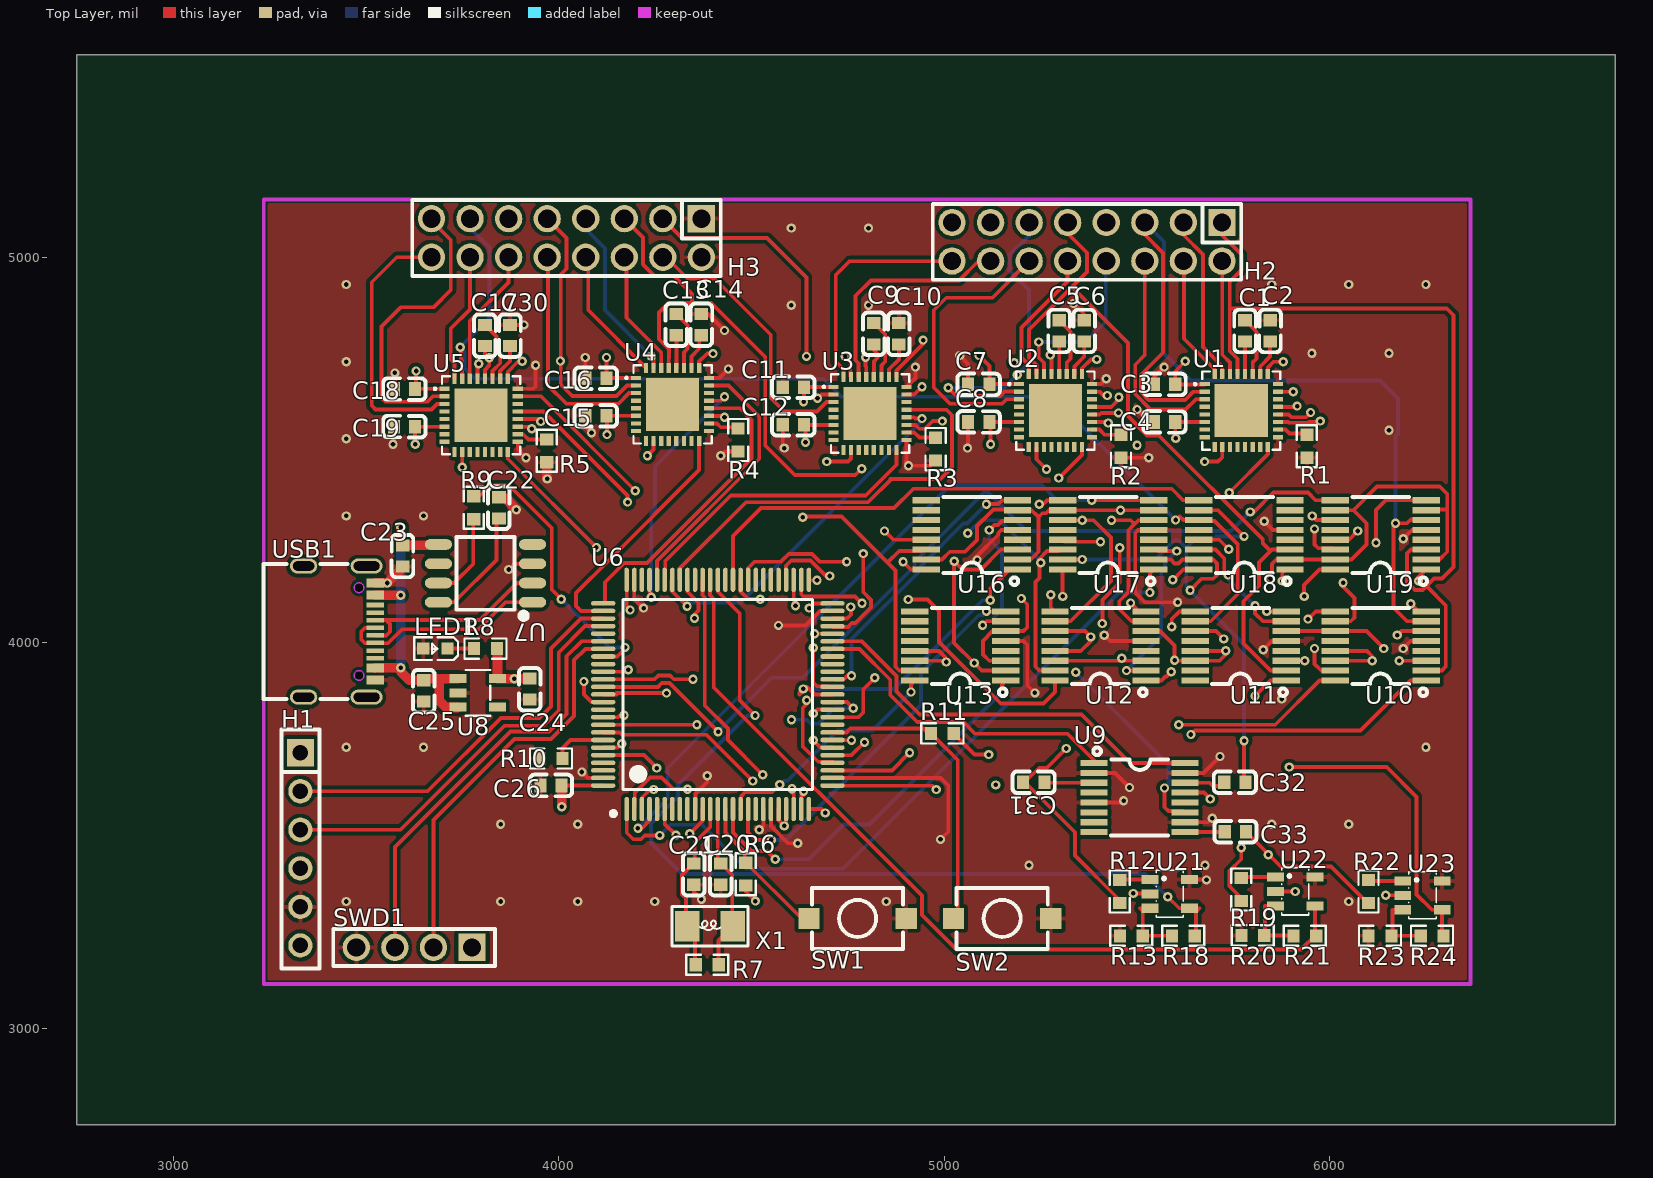
[diagram p0: Top Layer view]
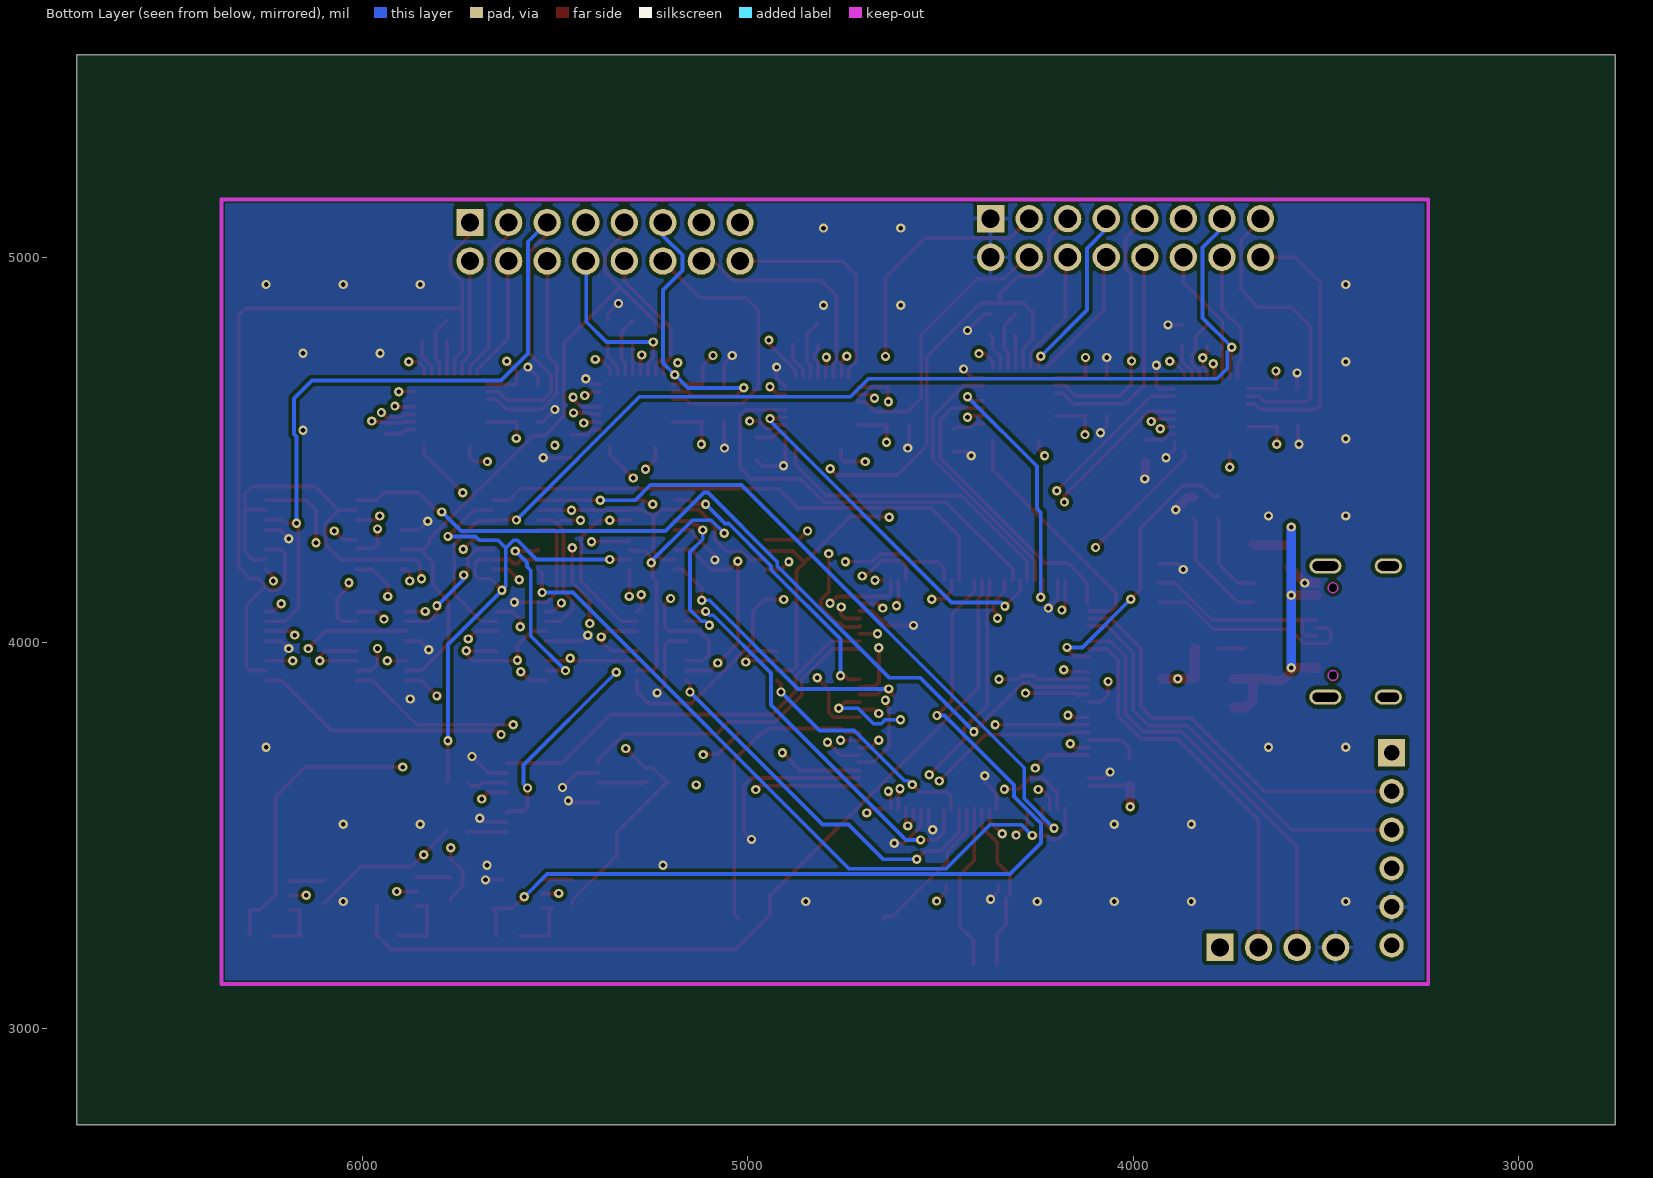
[diagram p1: Bottom Layer view, seen from below]
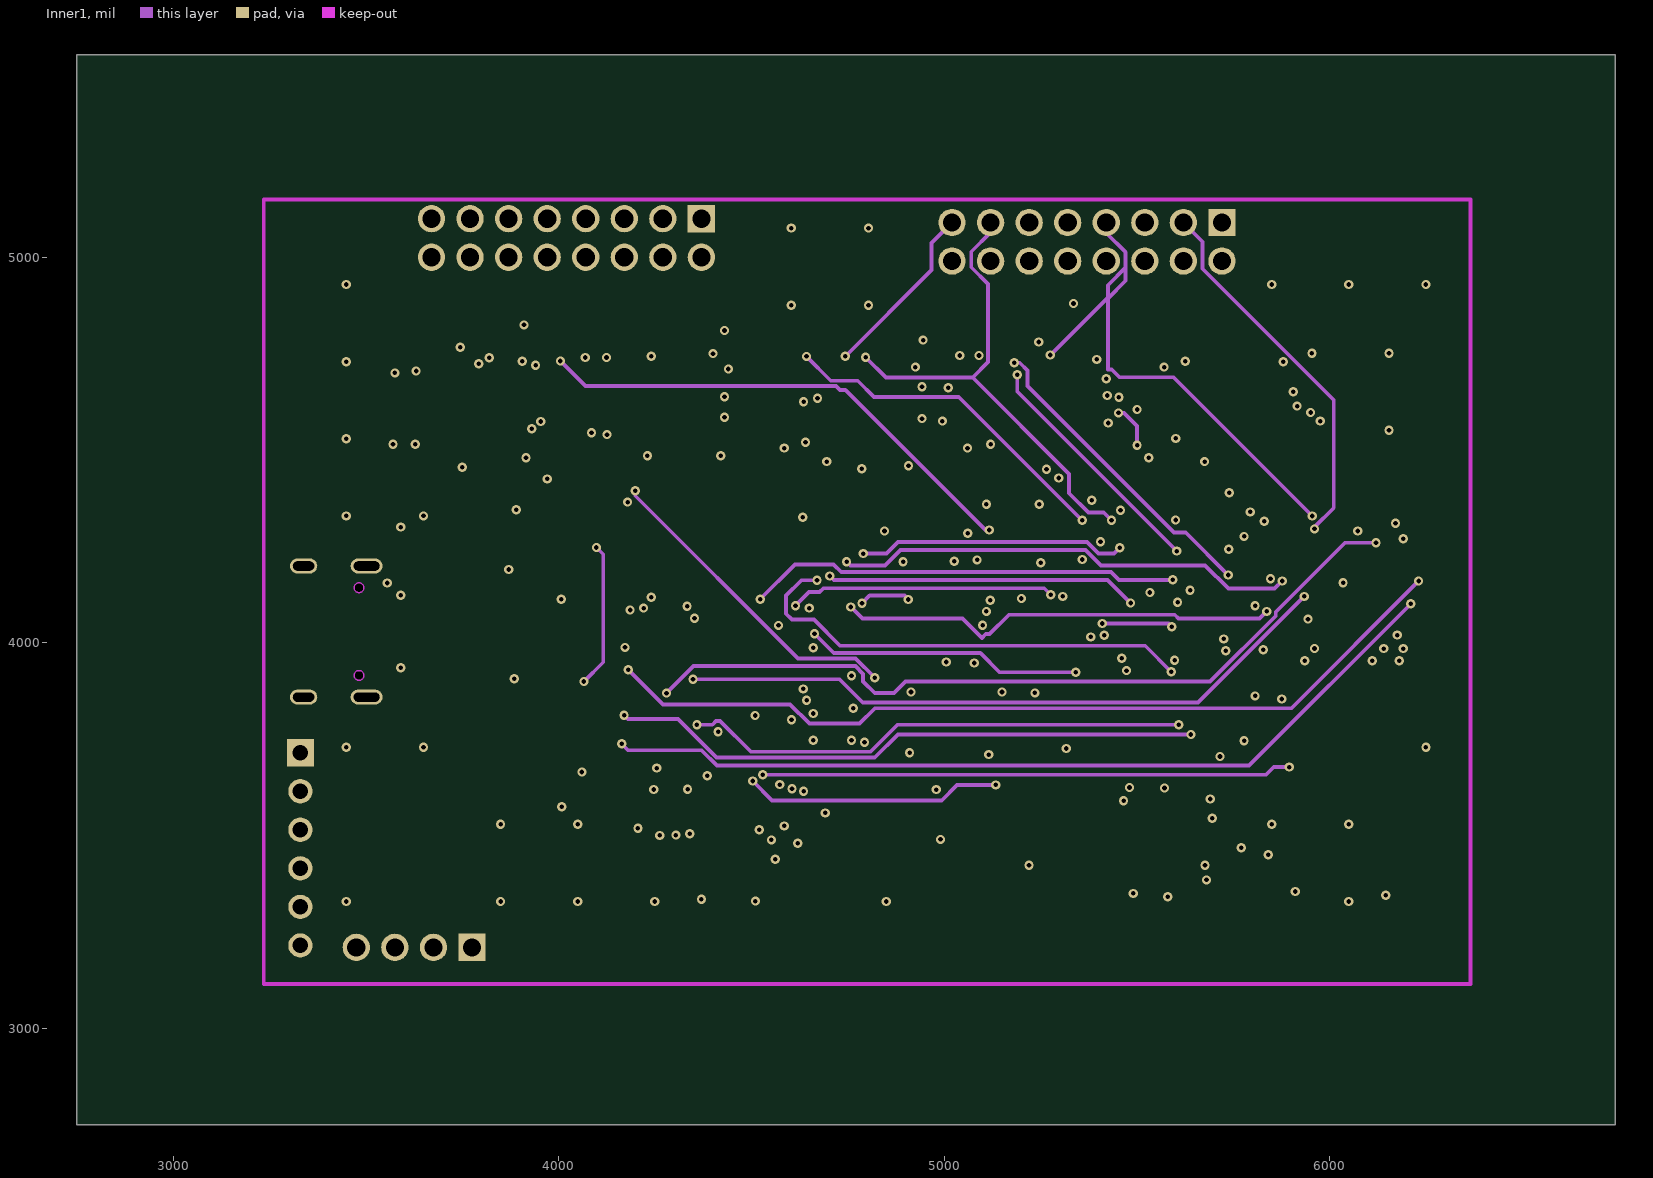
[diagram p2: Inner1]
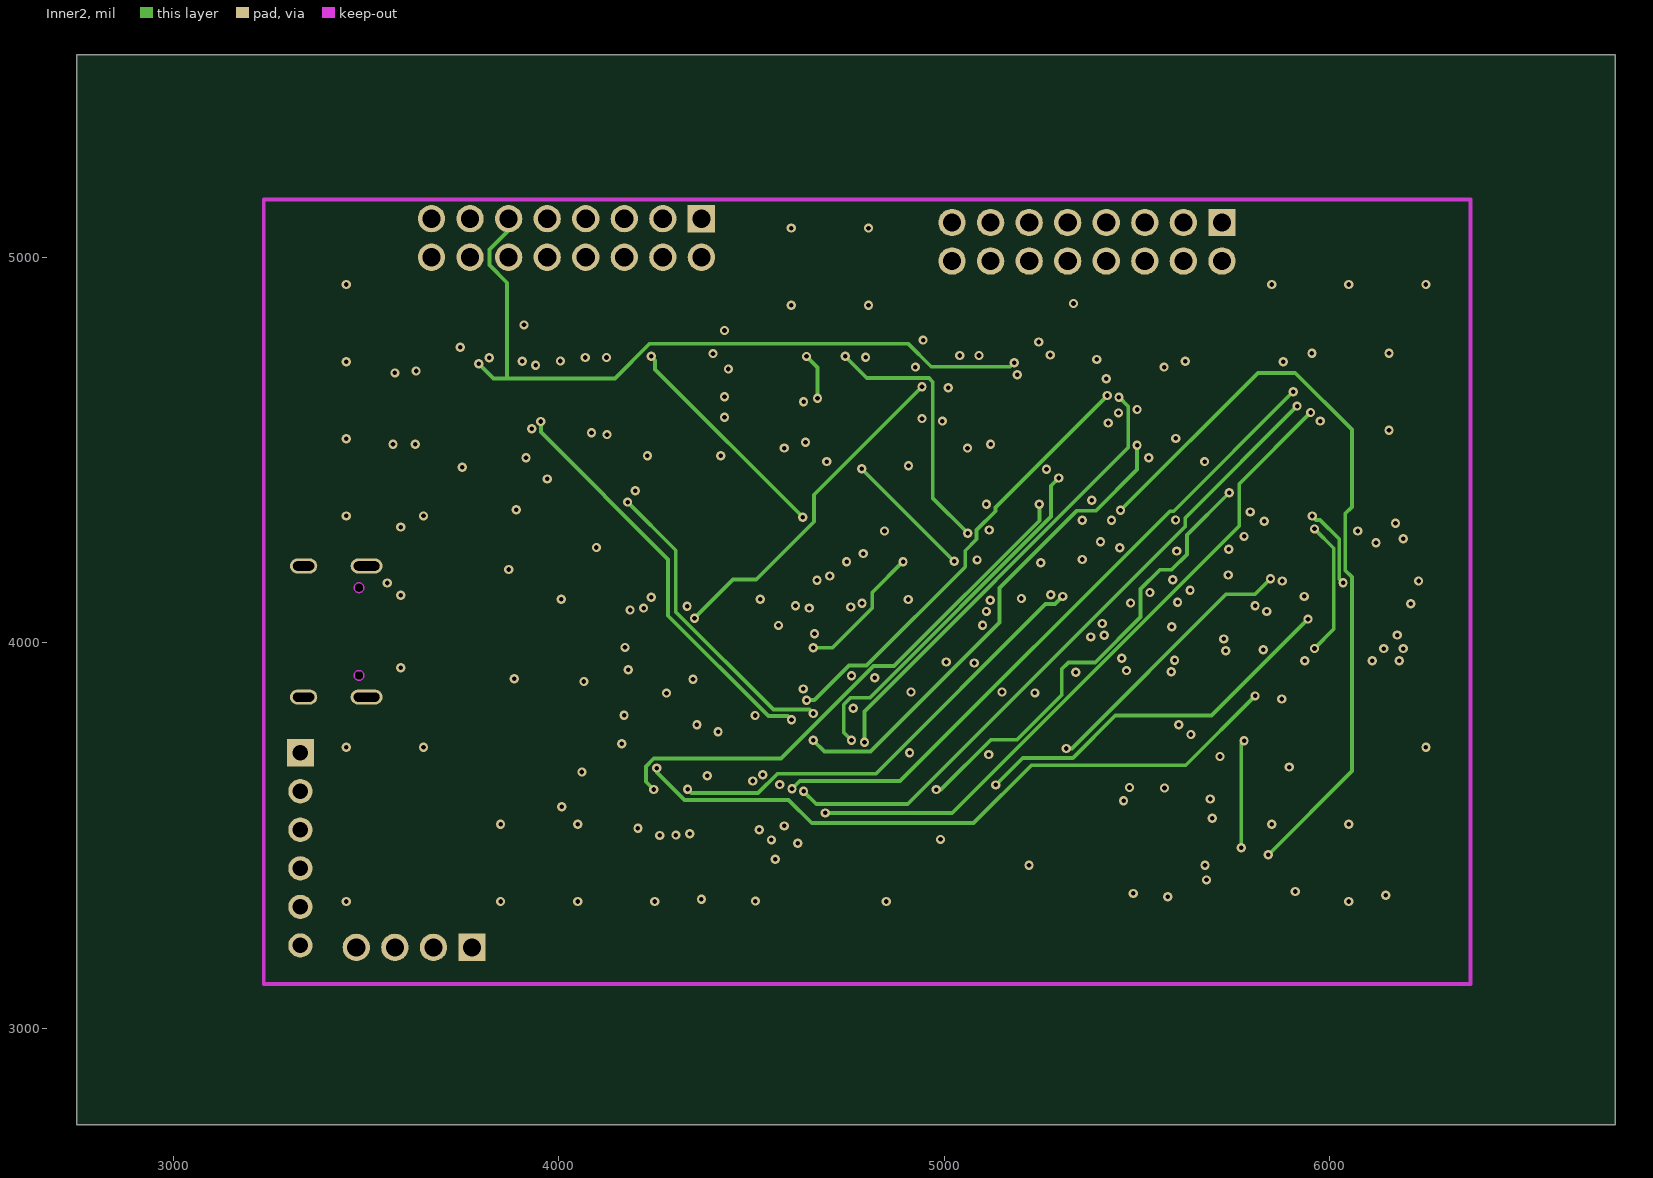
[diagram p3: Inner2]
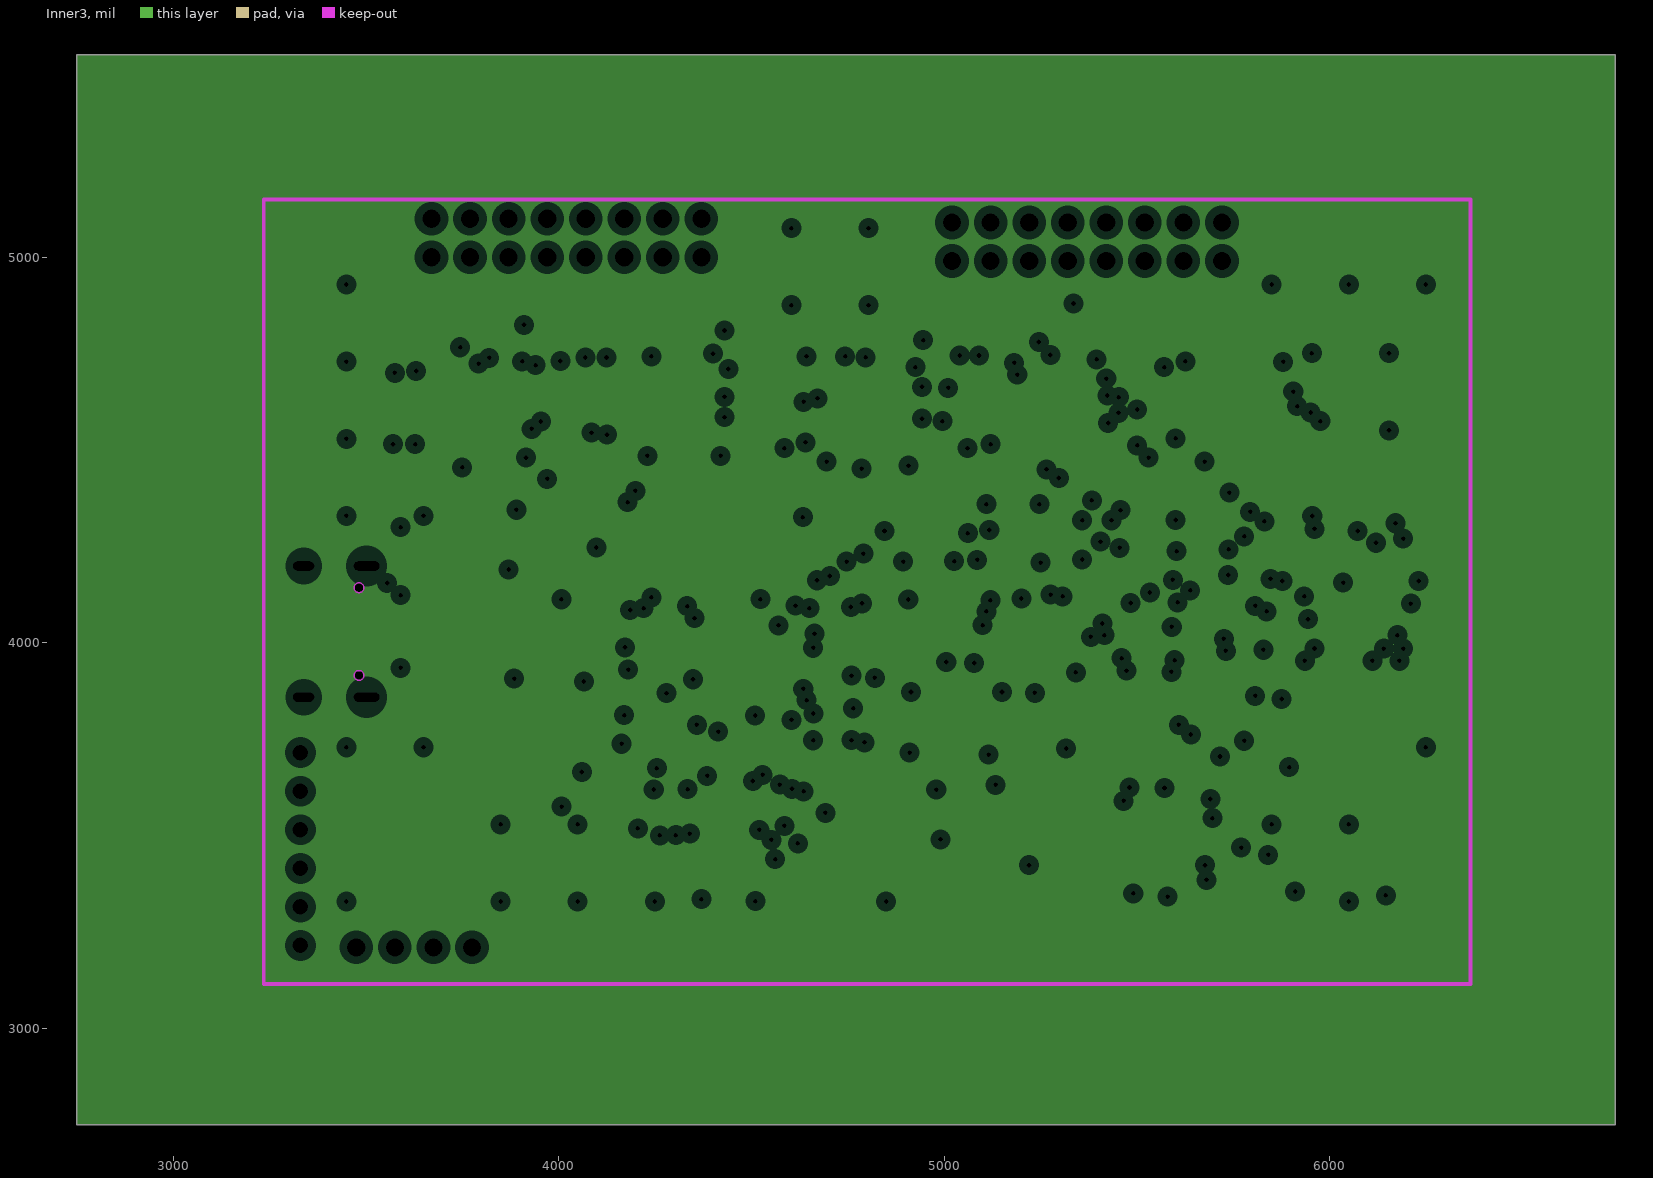
[diagram p4: Inner3, clearances drawn from the general rule]
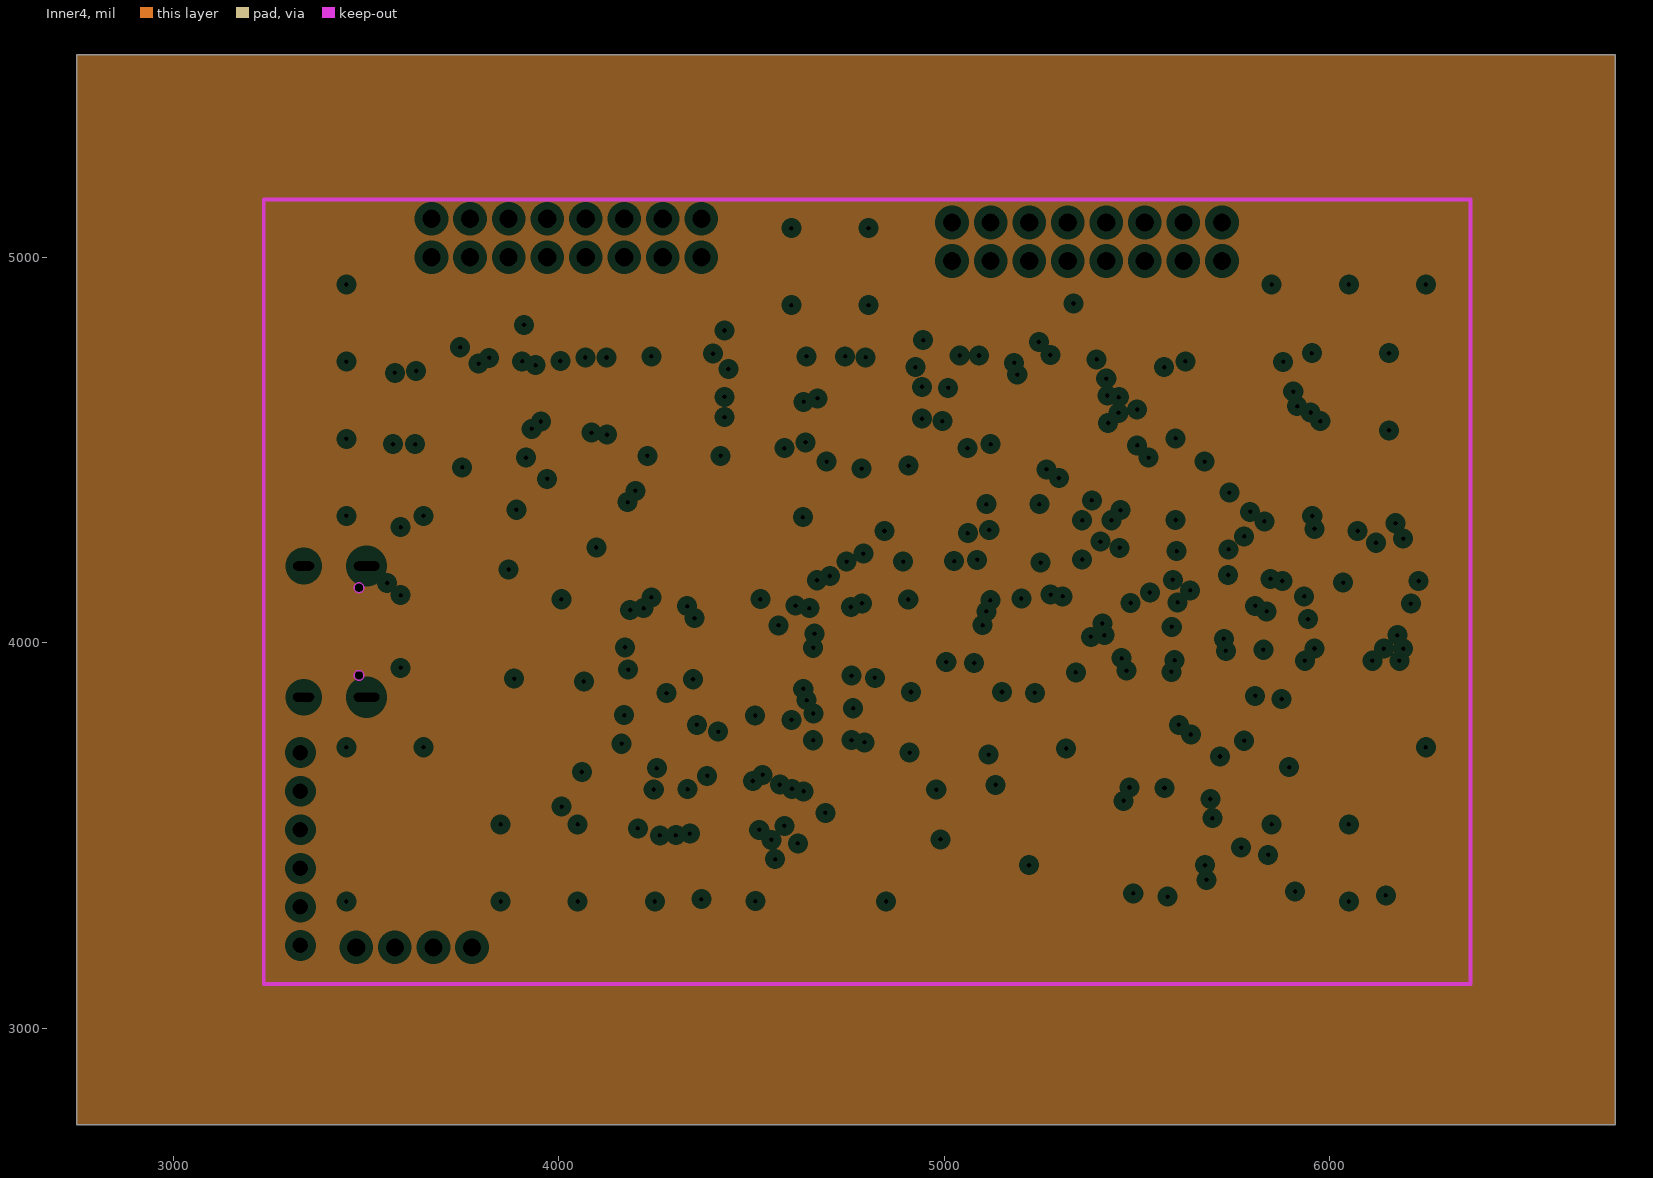
[diagram p5: Inner4, clearances drawn from the general rule]
# Altium PCB MISC49858.pcbdoc (part 1 of 3)
Units mil, origin at the board's own origin, x right, y up, seen from the top; angles counter-clockwise.
Board outline 3990 x 2775 mil, 6 copper layers (Top Layer, Inner1, Inner2, Inner3, Inner4, Bottom Layer), stack 60.565 mil thick; 79 components, 151 nets, 603 pads, 275 vias.

## Layer stack, top to bottom
Top Layer: signal copper 1.378
Dielectric1: surface 3.913, 3313 RC57% 4.2mil, Dk 0
Inner1: signal copper 0.598
Dielectric2: surface 21.654, 0.55mm H/H No copper, Dk 0
Inner2: signal copper 0.598
Dielectric3: surface 4.283, 2116 RC54% 4.9mil, Dk 0
Inner3: plane copper 0.598
Dielectric4: surface 21.654, 0.55mm H/H No copper, Dk 0
Inner4: plane copper 0.598
Dielectric5: surface 3.913, 3313 RC57% 4.2mil, Dk 0
Bottom Layer: signal copper 1.378

## Board outline
6740,2750 2750,2750 2750,5525 6740,5525

## Design rules (kind name [scope] priority, off if disabled: settings)
BoardOutlineClearance copperThickness2oz_1 [All] p2 off: genericclearance=7.99 ignorepadtopadclearanceinfootprint=FALSE except(0: Arc-SplitContinuation Track-SplitContinuation SMDPad-SplitContinuation THPad-SplitContinuation Via-SplitContinuation Fill-SplitContinuation Region-SplitContinuation Poly-SplitContinuation Text-SplitContinuation Hole-SplitContinuation; 5.98: SMDPad-CutoutEdge THPad-CutoutEdge Via-CutoutEdge Fill-CutoutEdge Region-CutoutEdge Text-CutoutEdge Hole-CutoutEdge; 10: Poly-OutlineEdge Poly-CutoutEdge; 11.81: Arc-OutlineEdge Track-OutlineEdge SMDPad-OutlineEdge THPad-OutlineEdge Via-OutlineEdge Fill-OutlineEdge Region-OutlineEdge Text-OutlineEdge Hole-OutlineEdge Arc-CutoutEdge Track-CutoutEdge)
BoardOutlineClearance Plane_innerPlane_1 [All] p4 off: genericclearance=4.02 ignorepadtopadclearanceinfootprint=FALSE except(0: Arc-SplitContinuation Track-SplitContinuation SMDPad-SplitContinuation THPad-SplitContinuation Via-SplitContinuation Fill-SplitContinuation Region-SplitContinuation Poly-SplitContinuation Text-SplitContinuation Hole-SplitContinuation; 5.98: SMDPad-CutoutEdge THPad-CutoutEdge Via-CutoutEdge Fill-CutoutEdge Region-CutoutEdge Text-CutoutEdge Hole-CutoutEdge; 10: Poly-OutlineEdge Poly-CutoutEdge; 11.81: Arc-OutlineEdge Track-OutlineEdge SMDPad-OutlineEdge THPad-OutlineEdge Via-OutlineEdge Fill-OutlineEdge Region-OutlineEdge Text-OutlineEdge Hole-OutlineEdge Arc-CutoutEdge Track-CutoutEdge)
BoardOutlineClearance Copper_copperRegion_1 [All] p6 off: genericclearance=4.02 ignorepadtopadclearanceinfootprint=FALSE except(0: Arc-SplitContinuation Track-SplitContinuation SMDPad-SplitContinuation THPad-SplitContinuation Via-SplitContinuation Fill-SplitContinuation Region-SplitContinuation Poly-SplitContinuation Text-SplitContinuation Hole-SplitContinuation; 5.98: SMDPad-CutoutEdge THPad-CutoutEdge Via-CutoutEdge Fill-CutoutEdge Region-CutoutEdge Text-CutoutEdge Hole-CutoutEdge; 10: Poly-OutlineEdge Poly-CutoutEdge; 11.81: Arc-OutlineEdge Track-OutlineEdge SMDPad-OutlineEdge THPad-OutlineEdge Via-OutlineEdge Fill-OutlineEdge Region-OutlineEdge Text-OutlineEdge Hole-OutlineEdge Arc-CutoutEdge Track-CutoutEdge)
BoardOutlineClearance copperThickness1oz_1 [All] p8: genericclearance=4.02 ignorepadtopadclearanceinfootprint=FALSE except(0: Arc-SplitContinuation Track-SplitContinuation SMDPad-SplitContinuation THPad-SplitContinuation Via-SplitContinuation Fill-SplitContinuation Region-SplitContinuation Poly-SplitContinuation Text-SplitContinuation Hole-SplitContinuation; 5.98: SMDPad-CutoutEdge THPad-CutoutEdge Via-CutoutEdge Fill-CutoutEdge Region-CutoutEdge Text-CutoutEdge Hole-CutoutEdge; 10: Poly-OutlineEdge Poly-CutoutEdge; 11.81: Arc-OutlineEdge Track-OutlineEdge SMDPad-OutlineEdge THPad-OutlineEdge Via-OutlineEdge Fill-OutlineEdge Region-OutlineEdge Text-OutlineEdge Hole-OutlineEdge Arc-CutoutEdge Track-CutoutEdge)
Clearance copperThickness2oz [All] p1 off: gap=7.99 ignorepadtopadclearanceinfootprint=FALSE except(5.98: SMDPad-Track SMDPad-SMDPad THPad-Track SMDPad-THPad THPad-THPad Track-Via SMDPad-Via THPad-Via Via-Via Fill-Track Region-Track Fill-SMDPad Region-SMDPad Fill-THPad Region-THPad Fill-Via Region-Via Fill-Fill Fill-Region Region-Region Arc-Track Arc-SMDPad Arc-THPad Arc-Via Fill-Arc Region-Arc Arc-Arc Text-Track SMDPad-Text Text-THPad Text-Via Fill-Text Region-Text Arc-Text Text-Text Hole-Track Hole-SMDPad Hole-THPad Hole-Via Fill-Hole Region-Hole Hole-Arc Hole-Text; 10: Poly-Track Poly-SMDPad Poly-THPad Poly-Via Poly-Fill Poly-Region Poly-Poly Poly-Arc Poly-Text Poly-Hole)
Clearance Plane_innerPlane [All] p3 off: gap=4.02 ignorepadtopadclearanceinfootprint=FALSE except(5.98: SMDPad-Track SMDPad-SMDPad THPad-Track SMDPad-THPad THPad-THPad Track-Via SMDPad-Via THPad-Via Via-Via Fill-Track Region-Track Fill-SMDPad Region-SMDPad Fill-THPad Region-THPad Fill-Via Region-Via Fill-Fill Fill-Region Region-Region Arc-Track Arc-SMDPad Arc-THPad Arc-Via Fill-Arc Region-Arc Arc-Arc Text-Track SMDPad-Text Text-THPad Text-Via Fill-Text Region-Text Arc-Text Text-Text Hole-Track Hole-SMDPad Hole-THPad Hole-Via Fill-Hole Region-Hole Hole-Arc Hole-Text; 10: Poly-Track Poly-SMDPad Poly-THPad Poly-Via Poly-Fill Poly-Region Poly-Poly Poly-Arc Poly-Text Poly-Hole)
Clearance Copper_copperRegion [All] p5 off: gap=4.02 ignorepadtopadclearanceinfootprint=FALSE except(5.98: SMDPad-Track SMDPad-SMDPad THPad-Track SMDPad-THPad THPad-THPad Track-Via SMDPad-Via THPad-Via Via-Via Fill-Track Region-Track Fill-SMDPad Region-SMDPad Fill-THPad Region-THPad Fill-Via Region-Via Fill-Fill Fill-Region Region-Region Arc-Track Arc-SMDPad Arc-THPad Arc-Via Fill-Arc Region-Arc Arc-Arc Text-Track SMDPad-Text Text-THPad Text-Via Fill-Text Region-Text Arc-Text Text-Text Hole-Track Hole-SMDPad Hole-THPad Hole-Via Fill-Hole Region-Hole Hole-Arc Hole-Text; 10: Poly-Track Poly-SMDPad Poly-THPad Poly-Via Poly-Fill Poly-Region Poly-Poly Poly-Arc Poly-Text Poly-Hole)
Clearance copperThickness1oz [All] p7: gap=4.02 ignorepadtopadclearanceinfootprint=FALSE except(5.98: SMDPad-Track SMDPad-SMDPad THPad-Track SMDPad-THPad THPad-THPad Track-Via SMDPad-Via THPad-Via Via-Via Fill-Track Region-Track Fill-SMDPad Region-SMDPad Fill-THPad Region-THPad Fill-Via Region-Via Fill-Fill Fill-Region Region-Region Arc-Track Arc-SMDPad Arc-THPad Arc-Via Fill-Arc Region-Arc Arc-Arc Text-Track SMDPad-Text Text-THPad Text-Via Fill-Text Region-Text Arc-Text Text-Text Hole-Track Hole-SMDPad Hole-THPad Hole-Via Fill-Hole Region-Hole Hole-Arc Hole-Text; 10: Poly-Track Poly-SMDPad Poly-THPad Poly-Via Poly-Fill Poly-Region Poly-Poly Poly-Arc Poly-Text Poly-Hole)
DiffPairsRouting differentialPair [All] p1: maxlimit=6 minlimit=6 mostfreqgap=6 toplayer_minwidth=5 toplayer_prefwidth=10 toplayer_maxwidth=100 toplayer_mingap=6 toplayer_prefgap=6 toplayer_maxgap=6 midlayer1_minwidth=5 midlayer1_prefwidth=10 midlayer1_maxwidth=100 midlayer1_mingap=6 midlayer1_prefgap=6 midlayer1_maxgap=6 midlayer2_minwidth=5 midlayer2_prefwidth=10 midlayer2_maxwidth=100 midlayer2_mingap=6 midlayer2_prefgap=6 midlayer2_maxgap=6 bottomlayer_minwidth=5 bottomlayer_prefwidth=10 bottomlayer_maxwidth=100 bottomlayer_mingap=6 bottomlayer_prefgap=6 bottomlayer_maxgap=6 maxuncoupledlength=10
HoleToHoleClearance otherClearance [All] p1: gap=11.8 allowstackedmicrovias=TRUE
Length netLength [All] p1: minlimit=0 maxlimit=0
PasteMaskExpansion pasteMaskExpansion [All] p1: expansion=0
PlaneConnect innerPlane [All] p1: planeconnectstyle=Relief reliefexpansion=20 reliefentries=4 reliefconductorwidth=10 reliefairgap=10
PolygonConnect copperRegion [(InNet('GND'))] p1: connectstyle=Relief reliefconductorwidth=10 reliefentries=4 polygonreliefangle="90 Angle" airgapwidth=10 via.connectstyle=Relief via.reliefconductorwidth=10 via.reliefentries=4 via.polygonreliefangle="90 Angle" via.airgapwidth=10
RoutingVias viaSize [All] p1: holewidth=12.01 width=24.02 viastyle="Through Hole" minholewidth=11.81 minwidth=19.68 maxholewidth=248.03 maxwidth=393.7
SolderMaskExpansion solderMaskExpansion [IsVia] p1: expansion=-1000 istentingtop=TRUE
SolderMaskExpansion solderMaskExpansion [All] p2: expansion=2 istentingtop=FALSE
Width copperThickness2oz_2 [All] p1 off: maxlimit=100 minlimit=8 preferedwidth=10
Width copperThickness1oz_2 [All] p2: maxlimit=100 minlimit=5 preferedwidth=10

## Components (designator, comment, footprint, x,y, rotation, side; value= is the part's Value field where it differs from the comment)
C1 "22pf/50V" C0603#1 5779.97,4809 r90 top
C2 "104" C0603#1 5844.97,4809 r90 top
C3 "10nF/25V" C0603#1 5571.38,4670.11 r0 top
C4 "4.7uF/50V" C0603#1 5571.38,4572.67 r0 top
C5 "4.7uF/50V" C0603#1 5297.87,4809 r90 top
C6 "104" C0603#1 5362.87,4809 r90 top
C7 "4.7uF/50V" C0603#1 5089.27,4670.11 r0 top
C8 "10nF/25V" C0603#1 5089.28,4572.67 r0 top
C9 "4.7uF/50V" C0603#1 4817.14,4801.62 r90 top
C10 "104" C0603#1 4882.14,4801.62 r90 top
C11 "4.7uF/50V" C0603#1 4608.55,4662.73 r0 top
C12 "10nF/25V" C0603#1 4608.55,4565.29 r0 top
C13 "4.7uF/50V" C0603#1 4305,4825 r90 top
C14 "104" C0603#1 4370,4825 r90 top
C15 "4.7uF/50V" C0603#1 4096.41,4588.67 r0 top
C16 "10nF/25V" C0603#1 4096.41,4686.11 r0 top
C17 "4.7uF/50V" C0603#1 3808.59,4796.94 r90 top
C18 "4.7uF/50V" C0603#1 3600,4658.05 r0 top
C19 "10nF/25V" C0603#1 3600,4560.61 r0 top
C20 "22pf" C0603#1 4420,3400 r90 top
C21 "22pf" C0603#1 4350,3400 r90 top
C22 "0.1UF" C0603#2 3845,4350 r90 top
C23 "0.1UF" C0603#2 3595,4225 r90 top
C24 "106" C0603#1 3925,3880 r90 top
C25 "106" C0603#1 3650,3875.12 r90 top
C26 "100nF" C0603#1 3980,3630 r0 top
C30 "104" C0603#1 3873.59,4796.94 r90 top
C31 "500uF" C0603#1 5231.81,3638.55 r180 top
C32 "500uF" C0603#1 5753.49,3638.55 r180 top
C33 "500uF" C0603#1 5755,3510 r180 top
H1 "" HDR-TH_6P-P2.54-V-F 3330,3465 r270 top
H2 "PZ254V-12-16P" HDR-TH_16P-P2.54-V-M-R2-C8-S2.54 5370,5040 r180 top
H3 "PZ254V-12-16P" HDR-TH_16P-P2.54-V-M-R2-C8-S2.54 4020,5050 r180 top
LED1 "19-217/R6C-AL1M2VY/3T" LED0603-RD 3680,3985 r180 top
R1 "470K/1%" R0603 5940.19,4509.77 r90 top
R2 "470K/1%" R0603 5458.08,4509.77 r90 top
R3 "470K/1%" R0603 4977.36,4502.39 r90 top
R4 "470K/1%" R0603 4465.22,4525.77 r90 top
R5 "470K/1%" R0603 3968.81,4497.71 r90 top
R6 "4.7k" R0603 4485,3400 r270 top
R7 "1M" R0603 4385,3165 r180 top
R8 "4.7k" R0603 3810,3985 r0 top
R9 "100R" R0603 3779.66,4350.34 r90 top
R10 "10K" R0603 3980,3700 r180 top
R11 "4.7k" R0603 4995,3765 r0 top
R12 "10K" R0603 5455,3355 r90 top
R13 "10K" R0603 5485,3240 r0 top
R18 "10K" R0603 5620,3240 r0 top
R19 "10K" R0603 5770,3360 r90 top
R20 "10K" R0603 5800.26,3241.02 r0 top
R21 "10K" R0603 5935,3240 r0 top
R22 "10K" R0603 6100,3355 r90 top
R23 "10K" R0603 6130,3240 r0 top
R24 "10K" R0603 6265,3240 r0 top
SW1 "YTS1C0191ABG00" SW-SMD_L6.0-W4.0-LS7.2 4775,3285 r180 top
SW2 "YTS1C0191ABG00" SW-SMD_L6.0-W4.0-LS7.2 5150,3285 r180 top
SWD1 "A2541HWV-4P" HDR-TH_4P-P2.54-V_A2541HWV-4P 3625,3210 r180 top
U1 "PCAP01AD" VQFN-32_L5.0-W5.0-P0.50-TL-EP 5770.19,4602.06 r0 top
U2 "PCAP01AD" VQFN-32_L5.0-W5.0-P0.50-TL-EP 5288.08,4602.06 r0 top
U3 "PCAP01AD" VQFN-32_L5.0-W5.0-P0.50-TL-EP 4807.36,4594.68 r0 top
U4 "PCAP01AD" VQFN-32_L5.0-W5.0-P0.50-TL-EP 4295.22,4618.06 r0 top
U5 "PCAP01AD" VQFN-32_L5.0-W5.0-P0.50-TL-EP 3798.81,4590 r0 top
U6 "STM32F103VET6" LQFP-100_L14.0-W14.0-P0.50-LS16.0-BL 4412.53,3865.99 r0 top
U7 "CH340N" SOP-8_150MIL 3810,4180 r180 top
U8 "RT9013-3.3GB" SOT-23-5_L2.9-W1.6-P0.94-LS2.8-BL 3790,3870 r270 top
U9 "TMUX1112PWR" TSSOP-16_L5.0-W4.4-P0.65-LS6.4-TL 5506.22,3598.55 r0 top
U10 "TMUX1112PWR" TSSOP-16_L5.0-W4.4-P0.65-LS6.4-TL 6131.88,3991.8 r180 top
U11 "TMUX1112PWR" TSSOP-16_L5.0-W4.4-P0.65-LS6.4-TL 5768.46,3991.8 r180 top
U12 "TMUX1112PWR" TSSOP-16_L5.0-W4.4-P0.65-LS6.4-TL 5405.04,3991.8 r180 top
U13 "TMUX1112PWR" TSSOP-16_L5.0-W4.4-P0.65-LS6.4-TL 5041.62,3991.8 r180 top
U16 "TMUX1112PWR" TSSOP-16_L5.0-W4.4-P0.65-LS6.4-TL 5071.62,4279.91 r180 top
U17 "TMUX1112PWR" TSSOP-16_L5.0-W4.4-P0.65-LS6.4-TL 5425.04,4279.91 r180 top
U18 "TMUX1112PWR" TSSOP-16_L5.0-W4.4-P0.65-LS6.4-TL 5778.46,4279.91 r180 top
U19 "TMUX1112PWR" TSSOP-16_L5.0-W4.4-P0.65-LS6.4-TL 6131.88,4279.91 r180 top
U21 "LMV321IDBVR" SOT-23-5_L3.0-W1.7-P0.95-LS2.8-BR 5584.72,3348.85 r180 top
U22 "LMV321IDBVR" SOT-23-5_L3.0-W1.7-P0.95-LS2.8-BR 5910,3355 r180 top
U23 "LMV321IDBVR" SOT-23-5_L3.0-W1.7-P0.95-LS2.8-BR 6240,3345 r180 top
USB1 "TYPE-C16PIN" USB-C-SMD_TYPE-C16PIN 3431.28,4029.1 r270 top
X1 "8MHz" SMD322522 4451.22,3265 r180 top

## Footprints (in the part's own frame and the unit in brackets; to place one, negate y for a bottom-side part, rotate by r counter-clockwise, add the part's x,y. Pads: shape width x height; smd on the part's side, far side on the other; paste and mask are expansions set on the pad)
C0603#1 [mm]
  rect 0.8x0.9 smd: 1(-0.7,0) 2(0.7,0)
  silkscreen extent -1.41,-0.71 1.39,0.72
C0603#2 [mm]
  rect 0.8x0.9 smd paste+0 mask+0.102: 1(-0.7,0) 2(0.7,0)
  silkscreen extent -1.4,-0.7 1.4,0.72
HDR-TH_4P-P2.54-V_A2541HWV-4P [mm]
  rect 1.8x1.8 hole 1.2: 1(-3.81,0)
  round 1.8 hole 1.2: 2(-1.27,0) 3(1.27,0) 4(3.81,0)
  silkscreen extent -5.33,-1.22 5.33,1.22
HDR-TH_6P-P2.54-V-F [mm]
  rect 1.8x1.8 hole 1.02: 1(-6.35,0)
  round 1.6 hole 1.02: 2(-3.81,0) 3(-1.27,0) 4(1.27,0) 5(3.81,0) 6(6.35,0)
  silkscreen extent -7.87,-1.25 7.87,1.25
HDR-TH_16P-P2.54-V-M-R2-C8-S2.54 [mm]
  rect 1.8x1.8 hole 1.2: 1(-8.89,-1.27)
  round 1.8 hole 1.2: 2(-8.89,1.27) 3(-6.35,-1.27) 4(-6.35,1.27) 5(-3.81,-1.27) 6(-3.81,1.27) 7(-1.27,-1.27) 8(-1.27,1.27) 9(1.27,-1.27) 10(1.27,1.27) 11(3.81,-1.27) 12(3.81,1.27) 13(6.35,-1.27) 14(6.35,1.27) 15(8.89,-1.27) 16(8.89,1.27)
  silkscreen extent -10.16,-2.5 10.16,2.5
LED0603-RD [mm]
  rect 0.8x0.8 smd: 1(-0.799,0) 2(0.799,0)
  silkscreen extent -1.49,-0.75 1.39,0.76
LQFP-100_L14.0-W14.0-P0.50-LS16.0-BL [mm]
  oval 0.3x1.6 smd: 1(-6,-7.55) 2(-5.5,-7.55) 3(-5,-7.55) 4(-4.5,-7.55) 5(-4,-7.55) 6(-3.5,-7.55) 7(-3,-7.55) 8(-2.5,-7.55) 9(-2,-7.55) 10(-1.5,-7.55) 11(-1,-7.55) 12(-0.5,-7.55) 13(0,-7.55) 14(0.5,-7.55) 15(1,-7.55) 16(1.5,-7.55) 17(2,-7.55) 18(2.5,-7.55) 19(3,-7.55) 20(3.5,-7.55) 21(4,-7.55) 22(4.5,-7.55) 23(5,-7.55) 24(5.5,-7.55) 25(6,-7.55) 51(6,7.55) 52(5.5,7.55) 53(5,7.55) 54(4.5,7.55) 55(4,7.55) 56(3.5,7.55) 57(3,7.55) 58(2.5,7.55) 59(2,7.55) 60(1.5,7.55) 61(1,7.55) 62(0.5,7.55) 63(0,7.55) 64(-0.5,7.55) 65(-1,7.55) 66(-1.5,7.55) 67(-2,7.55) 68(-2.5,7.55) 69(-3,7.55) 70(-3.5,7.55) 71(-4,7.55) 72(-4.5,7.55) 73(-5,7.55) 74(-5.5,7.55) 75(-6,7.55)
  oval 1.6x0.3 smd: 26(7.55,-6) 27(7.55,-5.5) 28(7.55,-5) 29(7.55,-4.5) 30(7.55,-4) 31(7.55,-3.5) 32(7.55,-3) 33(7.55,-2.5) 34(7.55,-2) 35(7.55,-1.5) 36(7.55,-1) 37(7.55,-0.5) 38(7.55,0) 39(7.55,0.5) 40(7.55,1) 41(7.55,1.5) 42(7.55,2) 43(7.55,2.5) 44(7.55,3) 45(7.55,3.5) 46(7.55,4) 47(7.55,4.5) 48(7.55,5) 49(7.55,5.5) 50(7.55,6) 76(-7.55,6) 77(-7.55,5.5) 78(-7.55,5) 79(-7.55,4.5) 80(-7.55,4) 81(-7.55,3.5) 82(-7.55,3) 83(-7.55,2.5) 84(-7.55,2) 85(-7.55,1.5) 86(-7.55,1) 87(-7.55,0.5) 88(-7.55,0) 89(-7.55,-0.5) 90(-7.55,-1) 91(-7.55,-1.5) 92(-7.55,-2) 93(-7.55,-2.5) 94(-7.55,-3) 95(-7.55,-3.5) 96(-7.55,-4) 97(-7.55,-4.5) 98(-7.55,-5) 99(-7.55,-5.5) 100(-7.55,-6)
  silkscreen extent -7.03,-8 6.25,6.25
R0603 [mil]
  rect 31.75x34.02 smd paste-3937.01 mask+2: 1(-29.66,0) 2(29.66,0)
  silkscreen extent -55,-26 55,26
SMD322522 [mm]
  rect 1.6x2 smd: 1(0,0) 2(3,0)
  silkscreen extent -1,-1.3 4,1.3
SOP-8_150MIL [mm]
  oval 1.8x0.7 smd: 1(-3.099,1.905) 2(-3.099,0.635) 3(-3.099,-0.635) 4(-3.099,-1.905) 5(3.099,-1.905) 6(3.099,-0.635) 7(3.099,0.635) 8(3.099,1.905)
  silkscreen extent -2.71,-2.4 1.91,2.99
SOT-23-5_L2.9-W1.6-P0.94-LS2.8-BL [mm]
  rect 0.6x1.1 smd paste+0 mask+0.05: 1(-0.94,-1.3) 2(0,-1.3) 3(0.94,-1.3) 4(0.94,1.3) 5(-0.94,1.3)
  silkscreen extent -1.51,-0.81 1.51,0.82
SOT-23-5_L3.0-W1.7-P0.95-LS2.8-BR [mm]
  rect 1.1x0.6 smd: 1(1.3,-0.95) 2(1.3,0) 3(1.3,0.95) 4(-1.3,0.95) 5(-1.3,-0.95)
  silkscreen extent -0.9,-1.55 0.9,1.55
SW-SMD_L6.0-W4.0-LS7.2 [mm]
  rect 1.4x1.4 smd paste+0 mask+0.05: 1(-3.2,0) 2(3.2,0)
  silkscreen extent -3,-2 3,2
TSSOP-16_L5.0-W4.4-P0.65-LS6.4-TL [mil]
  rect 71x16 smd: 1(-118.11,89.57) 2(-118.11,63.97) 3(-118.11,38.38) 4(-118.11,12.79) 5(-118.11,-12.8) 6(-118.11,-38.39) 7(-118.11,-63.98) 8(-118.11,-89.57) 9(118.11,-89.57) 10(118.11,-63.98) 11(118.11,-38.39) 12(118.11,-12.8) 13(118.11,12.79) 14(118.11,38.38) 15(118.11,63.97) 16(118.11,89.57)
  silkscreen extent -120,-98 74,130
USB-C-SMD_TYPE-C16PIN [mm]
  oval 1x2.1 hole 0.6 slot 1.7 at 90 deg: 1(-4.32,1.787) 2(4.32,1.787)
  oval 1x1.8 hole 0.6 slot 1.4 at 90 deg: 3(-4.32,-2.362) 4(4.32,-2.362)
  rect 0.6x1.15 smd paste-100 mask+0.051: A1B12(-3.2,2.362) A4B9(-2.4,2.362) B1A12(3.2,2.362) B4A9(2.4,2.362)
  rect 0.3x1.15 smd paste-100 mask+0.051: A5(-1.25,2.362) A6(-0.25,2.362) A7(0.25,2.362) A8(1.25,2.362) B5(1.75,2.362) B6(0.75,2.362) B7(-0.75,2.362) B8(-1.75,2.362)
  Board Outline Layer circle w0.003: c2.89,1.288 r0.325
  Board Outline Layer circle w0.003: c-2.89,1.288 r0.325
  Board Outline Layer region: 2.89,1.613 3.031,1.581 3.144,1.491 3.207,1.36 3.207,1.216 3.144,1.085 3.031,0.995 2.89,0.963 2.89,0.963 2.749,0.995 2.636,1.085 2.573,1.216 2.573,1.36 2.636,1.491 2.749,1.581 2.89,1.613
  Board Outline Layer region: 2.89,1.613 2.968,1.604 3.041,1.576 3.106,1.531 3.157,1.473 3.194,1.403 3.213,1.327 3.213,1.249 3.194,1.173 3.157,1.103 3.106,1.045 3.041,1 2.968,0.972 2.89,0.963 2.812,0.972 2.739,1 2.675,1.045 2.623,1.103 2.586,1.173 2.567,1.249 2.567,1.327 2.586,1.403 2.623,1.473 2.675,1.531 2.739,1.576 2.812,1.604
  Board Outline Layer region: -2.89,1.613 -2.749,1.581 -2.636,1.491 -2.573,1.36 -2.573,1.216 -2.636,1.085 -2.749,0.995 -2.89,0.963 -2.89,0.963 -3.031,0.995 -3.144,1.085 -3.207,1.216 -3.207,1.36 -3.144,1.491 -3.031,1.581 -2.89,1.613
  Board Outline Layer region: -2.89,1.613 -2.812,1.604 -2.739,1.576 -2.675,1.531 -2.623,1.473 -2.586,1.403 -2.567,1.327 -2.567,1.249 -2.586,1.173 -2.623,1.103 -2.675,1.045 -2.739,1 -2.812,0.972 -2.89,0.963 -2.968,0.972 -3.041,1 -3.106,1.045 -3.157,1.103 -3.194,1.173 -3.213,1.249 -3.213,1.327 -3.194,1.403 -3.157,1.473 -3.106,1.531 -3.041,1.576 -2.968,1.604
  Multi-Layer board cut-out: 2.89,1.613 3.031,1.581 3.144,1.491 3.207,1.36 3.207,1.216 3.144,1.085 3.031,0.995 2.89,0.963 2.89,0.963 2.749,0.995 2.636,1.085 2.573,1.216 2.573,1.36 2.636,1.491 2.749,1.581 2.89,1.613
  Multi-Layer board cut-out: -2.89,1.613 -2.749,1.581 -2.636,1.491 -2.573,1.36 -2.573,1.216 -2.636,1.085 -2.749,0.995 -2.89,0.963 -2.89,0.963 -3.031,0.995 -3.144,1.085 -3.207,1.216 -3.207,1.36 -3.144,1.491 -3.031,1.581 -2.89,1.613
  silkscreen extent -4.45,-5 4.45,0.52
VQFN-32_L5.0-W5.0-P0.50-TL-EP [mm]
  rect 0.665x0.28 smd paste-100 mask+0.051: 1(-2.407,1.75) 2(-2.407,1.25) 3(-2.407,0.75) 4(-2.407,0.25) 5(-2.407,-0.25) 6(-2.407,-0.75) 7(-2.407,-1.25) 8(-2.407,-1.75) 17(2.407,-1.75) 18(2.407,-1.25) 19(2.407,-0.75) 20(2.407,-0.25) 21(2.407,0.25) 22(2.407,0.75) 23(2.407,1.25) 24(2.407,1.75)
  rect 0.28x0.665 smd paste-100 mask+0.051: 9(-1.75,-2.407) 10(-1.25,-2.407) 11(-0.75,-2.407) 12(-0.25,-2.407) 13(0.25,-2.407) 14(0.75,-2.407) 15(1.25,-2.407) 16(1.75,-2.407) 25(1.75,2.407) 26(1.25,2.407) 27(0.75,2.407) 28(0.25,2.407) 29(-0.25,2.407) 30(-0.75,2.407) 31(-1.25,2.407) 32(-1.75,2.407)
  rect 3.5x3.5 smd paste-100 mask+0.051: 33(0,0)
  silkscreen extent -3.11,-2.58 2.58,2.58

## Via types
v1: diameter 24.02, hole 12, Top Layer to Bottom Layer, 275 vias

## Nets (pads, with @x,y where several pads share a name; then routed paths per layer and width w, separated by ;. In a path a pad name is that pad's centre, name@x,y a point inside that pad or via, vN(x,y) a via of type N, cw(c..) or ccw(c..) an arc to the next point about the centre after c; other vN are vias at no path point)
3V3: C3.2 C4.2 C7.2 C8.2 C11.2 C12.2 C15.2 C16.2 C18.2 C19.2 C24.2 C26.2 H1.4 R6.2 R8.2 R11.2 SWD1.1 U1.1 U1.6 U1.10 U1.19 U1.25 U2.1 U2.6 U2.10 U2.19 U2.25 U3.1 U3.6 U3.10 U3.19 U3.25 U4.1 U4.6 U4.10 U4.19 U4.25 U5.1 U5.6 U5.10 U5.19 U5.25 U6.6 U6.11 U6.21 U6.22 U6.28 U6.50 U6.75 U6.100 U8.5 U9.13 U10.3 U10.6 U10.11 U10.13 U10.14 U11.3 U11.6 U11.11 U11.13 U11.14 U12.3 U12.6 U12.11 U12.13 U12.14 U13.3 U13.6 U13.13 U13.14 U16.13 U17.13 U18.13 U19.13 U21.2 U22.2 U23.2 | length 6100
  Top Layer w9.92: v1(3627.56,4515) C19.2@3627.56,4560.61 3627.7,4560.47 U5.6@3704.03,4560.47 ; C18.2@3627.56,4658.05 C18.2@3628.41,4658.9 ; v1(3630,4705) 3630,4660.49 C18.2@3628.41,4658.9 ; U5.1@3704.03,4658.9 C18.2@3628.41,4658.9 ; v1(3749.6,4455) U5.10@3749.6,4495.22 ; U5.25@3867.71,4684.78 3867.71,4702.71 3895,4730 v1(3905,4730) ; U5.19@3893.59,4560.47 3924.53,4560.47 v1(3930,4555) ; v1(4123.97,4740) C16.2@4123.97,4686.11 4124.82,4686.96 U4.1@4200.44,4686.96 ; v1(4125,4540) 4125,4587.64 C15.2@4123.97,4588.67 4200.3,4588.67 U4.6@4200.44,4588.53 ; U6.75@4176.31,4163.23 4176.31,4093.69 v1(4185,4085) ; v1(4230,4485) 4246.01,4501.01 U4.10@4246.01,4523.28 ; U4.25@4364.12,4712.84 4364.12,4729.12 4385,4750 v1(4400,4750) ; C11.2@4636.11,4662.73 4636.97,4663.58 U3.1@4712.58,4663.58 ; C8.2@5116.84,4572.67 5120,4569.51 v1(5120,4515) ; U13.3@5159.72,3953.42 5116.58,3953.42 5100,3970 5100,4005 5125.19,4030.19 U13.6@5159.72,4030.19 ; U2.10@5238.87,4507.28 5238.87,4476.13 v1(5265,4450) ; U12.14@5286.92,3953.42 5453.42,3953.42 v1(5460,3960) 5466.58,3953.42 U12.3@5523.14,3953.42 ; U12.13@5286.92,3979.01 5354.01,3979.01 5380,4005 v1(5380,4015.22) 5365.03,4030.19 U12.11@5286.92,4030.19 ; U2.19@5382.86,4572.53 5422.47,4572.53 v1(5425,4570) ; v1(5490,3350) 5532.39,3350 U21.2@5533.53,3348.85 ; U12.6@5523.14,4030.19 5559.81,4030.19 5597.27,3992.73 v1(5597.27,3954.7) 5598.56,3953.42 U11.14@5650.34,3953.42 5713.42,3953.42 5730,3970 v1(5730,3979.01) U11.13@5650.34,3979.01 ; v1(5600,4530) 5598.94,4531.06 C4.2@5598.94,4572.67 5675.27,4572.67 U1.6@5675.41,4572.53 ; U9.13@5624.33,3611.34 5673.66,3611.34 v1(5690,3595) ; v1(5625,4730) 5598.94,4703.94 C3.2@5598.94,4670.11 5674.55,4670.11 U1.1@5675.41,4670.96 ; U11.11@5650.34,4030.19 5704.81,4030.19 v1(5725,4010) ; U18.13@5660.34,4267.12 5712.88,4267.12 v1(5737.6,4242.4) ; v1(5675,4470) 5710,4470 5720.98,4480.98 U1.10@5720.98,4507.28 ; U1.25@5839.09,4696.84 5839.09,4714.09 5853.77,4728.77 v1(5878.77,4728.77) ; U22.2@5858.81,3355 v1(5910,3355) ; U1.19@5864.97,4572.53 5892.08,4572.53 5894.03,4570.58 5943.71,4570.58 5945.67,4572.53 5972.53,4572.53 v1(5975,4575) ; U11.3@5886.56,3953.42 v1(5935,3953.42) ; U11.6@5886.56,4030.19 U10.11@6013.76,4030.19 6094.81,4030.19 v1(6140,3985) ; U10.14@6013.76,3953.42 v1(6110,3953.42) 6110,3965 6095.99,3979.01 U10.13@6013.76,3979.01 ; v1(6145,3345) U23.2@6188.81,3345 ; v1(6175,4020) 6185.19,4030.19 U10.6@6249.98,4030.19 ; v1(6180,3953.42) U10.3@6249.98,3953.42
  Top Layer w10: C26.2@4007.56,3630 4007.79,3629.77 U6.100@4115.29,3629.77 ; U6.6@4274.73,3568.75 4274.73,3530.27 v1(4303.79,3501.21) ; v1(4340,3505) 4373.16,3538.16 U6.11@4373.16,3568.75 ; U4.19@4390,4588.53 4426.47,4588.53 v1(4430,4585) ; R6.2@4485,3370.34 4485,3355 v1(4510,3330) ; U6.21@4570.01,3568.75 4570.01,3540 v1(4585.01,3525) 4589.7,3529.69 U6.22@4589.7,3568.75 ; v1(4635,4625) 4636.11,4626.11 C11.2@4636.11,4662.73 ; v1(4640,4520) 4640,4561.4 C12.2@4636.11,4565.29 4712.44,4565.29 U3.6@4712.58,4565.15 ; v1(4650,4090) 4662.21,4102.21 U6.50@4709.77,4102.21 ; v1(4695,4470) 4750,4470 4758.15,4478.15 U3.10@4758.15,4499.9 ; U6.28@4709.77,3669.14 4864.14,3669.14 v1(4910,3715) ; v1(4845,4290) 4867.88,4267.12 U16.13@4953.5,4267.12 ; U3.25@4876.26,4689.46 4876.26,4706.26 4945,4775 v1(4945,4785) ; U3.19@4902.14,4565.15 4924.85,4565.15 4935,4555 4950,4555 4970,4575 v1(4995,4575) ; U13.14@4923.5,3953.42 v1@5001.58,3953.42 ; U13.13@4923.5,3979.01 4985.99,3979.01 5001.58,3963.42 v1@5001.58,3953.42 ; v1(5005,3950) v1@5001.58,3953.42 ; R11.2@5024.66,3765 5024.66,3763.87 5078.53,3710 v1(5115,3710) ; v1(5090,4745) 5116.83,4718.17 C7.2@5116.83,4670.11 5117.69,4670.96 U2.1@5193.3,4670.96 ; C8.2@5116.84,4572.67 5193.16,4572.67 U2.6@5193.3,4572.53 ; U13.6@5159.72,4030.19 5205.19,4030.19 5215,4040 5215,4100 v1(5200,4115) ; U17.13@5306.92,4267.12 5311.92,4262.12 v1(5405,4262.12) ; U2.25@5356.98,4696.84 5356.98,4711.98 5380,4735 v1(5395,4735) ; U19.13@6013.76,4267.12 6049.13,4267.12 v1(6072.01,4290)
  Top Layer w25: R8.2@3839.66,3985 3841.19,3983.47 U8.5@3841.19,3907.01 v1(3884.47,3907.01) 3924.45,3907.01 C24.2@3925,3907.56 ; v1(4007.56,3575) C26.2@4007.56,3630
$2N131: U7.1 USB1.A6 USB1.B6 | length 556.6
  Top Layer w10: USB1.B6@3524.29,3999.57 USB1.B6@3527.63,3998.94 ; USB1.A6@3524.29,4038.94 3497.63,4038.94 3487.63,4028.94 3487.63,4008.94 3497.63,3998.94 3557.63,3998.94 3593.68,4035 3791.57,4035 3861.57,4105 U7.1@3932,4105